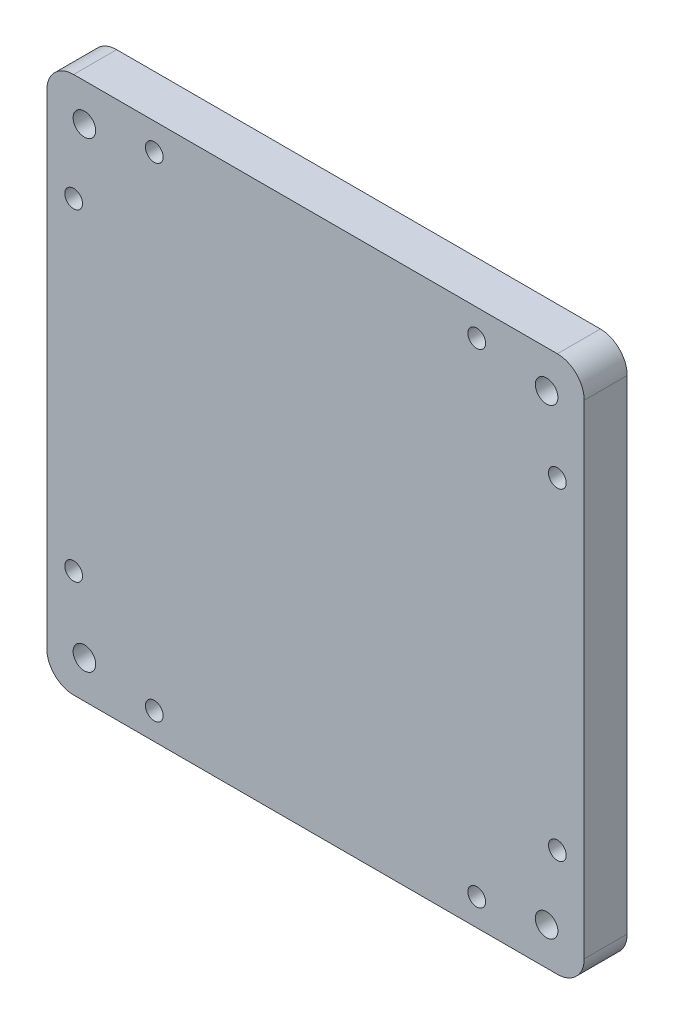
SolidWorks part; units mm, degrees
ref_plane "Front Plane" through (0, 0, 0) normal (0, 0, 1) x (1, 0, 0)
ref_plane "Top Plane" through (0, 0, 0) normal (0, 1, 0) x (1, 0, 0)
ref_plane "Right Plane" through (0, 0, 0) normal (1, 0, 0) x (0, 0, -1)
other "Configuration Table"
sketch "Sketch1" plane through (0, 0, 0) normal (0, 0, 1) x (1, 0, 0)
  line L1 (-45, 50) -> (45, 50)
  line L2 (-50, 45) -> (-50, -45)
  line L3 (-45, -50) -> (45, -50)
  line L4 (50, 45) -> (50, -45)
  line L5 (-50, 50) -> (50, -50) construction
  line L6 (-50, -50) -> (50, 50) construction
  arc A0 (45, -50) -> (50, -45) centre (45, -45) ccw
  arc A1 (-50, -45) -> (-45, -50) centre (-45, -45) ccw
  arc A2 (45, 50) -> (50, 45) centre (45, 45) cw
  arc A3 (-45, 50) -> (-50, 45) centre (-45, 45) ccw
  point P0 (0, 0)
  dimension "D3" = 5
  dimension "D1" = 100
  dimension "D2" = 100
extrude "Boss-Extrude1" add sketch "Sketch1" along normal blind 8
sketch "Sketch2" plane through (0, 0, 8) normal (0, 0, 1) x (1, 0, 0)
  line L1 (-43, 43) -> (43, 43) construction
  line L2 (-43, 43) -> (-43, -43) construction
  line L3 (-43, -43) -> (43, -43) construction
  line L4 (43, 43) -> (43, -43) construction
  line L5 (-43, 43) -> (43, -43) construction
  line L6 (-43, -43) -> (43, 43) construction
  circle A0 centre (0, 0) radius 27.3626 construction
  point P0 (0, 0)
  dimension "D1" = 86
  dimension "D2" = 86
hole_wizard "M5 Tapped Hole1" positions "3DSketch1" profile "Sketch3" tap size "M5" standard "GB"
sketch3d "3DSketch1"
  point P0 (-43, 43, 8)
  point P3 (43, 43, 8)
  point P6 (43, -43, 8)
  point P9 (-43, -43, 8)
sketch "Sketch3" plane through (-43, 43, 8) normal (1, 0, 0) x (0, -1, 0)
  line L0 (0, 0) -> (0, 13.6618)
  line L1 (0, 13.6618) -> (2.1, 12.4)
  line L2 (2.1, 12.4) -> (2.1, 0)
  line L5 (2.1, 0) -> (0, 0)
  line L10 (0, 13.6618) -> (-2.1, 12.4) construction
  line L11 (0, -6.35) -> (0, 107.95) construction
  dimension "螺纹孔钻头直径" = 4.2
  dimension "螺纹孔钻头深度" = 12.4
  dimension "导头角度" = 118
cosmetic thread "Hole Thread Line 1" parameters "D1"=10, "D2"=5
cosmetic thread "Hole Thread Line 2" parameters "D1"=10, "D2"=5
cosmetic thread "Hole Thread Line 3" parameters "D1"=10, "D2"=5
cosmetic thread "Hole Thread Line 4" parameters "D1"=10, "D2"=5
sketch "Sketch4" plane through (0, 0, 8) normal (0, 0, 1) x (1, 0, 0)
  line L0 (-45, -50) -> (45, -50) construction
  line L1 (-45, 45) -> (45, 45) construction
  line L2 (-45, 45) -> (-45, -45) construction
  line L3 (-45, -45) -> (45, -45) construction
  line L4 (45, 45) -> (45, -45) construction
  line L5 (-45, 45) -> (45, -45) construction
  line L6 (-45, -45) -> (45, 45) construction
  line L7 (50, -45) -> (50, 45) construction
  line L8 (0, 0) -> (0, -50) construction
  line L9 (-30, -45) -> (-30, -36.3734) construction
  line L10 (30, -45) -> (30, -36.6885) construction
  line L11 (-45, 30) -> (-36.3734, 30) construction
  line L12 (-45, -30) -> (-36.6885, -30) construction
  line L13 (30, 45) -> (30, 36.3734) construction
  line L14 (-30, 45) -> (-30, 36.6885) construction
  line L15 (45, -30) -> (36.3734, -30) construction
  line L16 (45, 30) -> (36.6885, 30) construction
  circle A0 centre (0, 0) radius 27.3626 construction
  point P0 (0, 0)
  point P31 (0, 0)
  point P42 (0, 0)
  dimension "D1" = 5
  dimension "D2" = 5
  dimension "D3" = 60
  dimension "D4" = 30
  dimension "D5" = 4
hole_wizard "M4 Tapped Hole1" positions "3DSketch2" profile "Sketch5" tap size "M4" standard "GB"
sketch3d "3DSketch2"
  point P0 (-30, -45, 8)
  point P3 (30, -45, 8)
  point P7 (-45, -30, 8)
  point P10 (-45, 30, 8)
  point P13 (45, 30, 8)
  point P16 (45, -30, 8)
  point P19 (-30, 45, 8)
  point P22 (30, 45, 8)
sketch "Sketch5" plane through (-30, -45, 8) normal (1, 0, 0) x (0, -1, 0)
  line L0 (0, 0) -> (0, 11.0914)
  line L1 (0, 11.0914) -> (1.65, 10.1)
  line L2 (1.65, 10.1) -> (1.65, 0)
  line L5 (1.65, 0) -> (0, 0)
  line L10 (0, 11.0914) -> (-1.65, 10.1) construction
  line L11 (0, -6.35) -> (0, 107.95) construction
  dimension "螺纹孔钻头直径" = 3.3
  dimension "螺纹孔钻头深度" = 10.1
  dimension "导头角度" = 118
cosmetic thread "Hole Thread Line 5" parameters "D1"=8, "D2"=4
cosmetic thread "Hole Thread Line 6" parameters "D1"=8, "D2"=4
cosmetic thread "Hole Thread Line 7" parameters "D1"=8, "D2"=4
cosmetic thread "Hole Thread Line 8" parameters "D1"=8, "D2"=4
cosmetic thread "Hole Thread Line 9" parameters "D1"=8, "D2"=4
cosmetic thread "Hole Thread Line 10" parameters "D1"=8, "D2"=4
cosmetic thread "Hole Thread Line 11" parameters "D1"=8, "D2"=4
cosmetic thread "Hole Thread Line 12" parameters "D1"=8, "D2"=4
